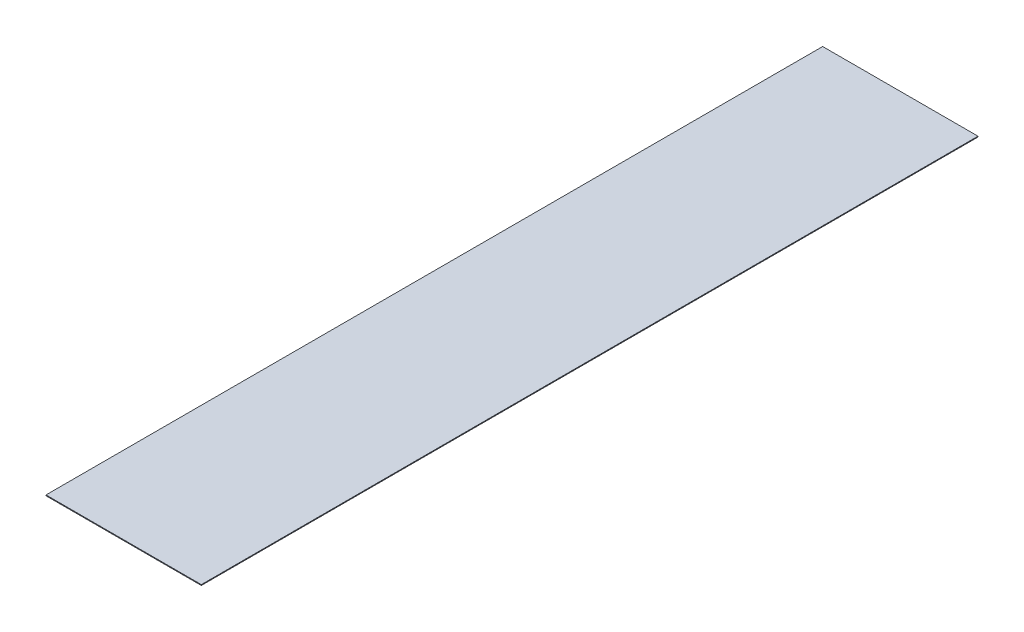
from build123d import *

# Parameters (mm, degrees)
SKETCH1_W           = 200
SKETCH1_H           = 1000
BOSS_EXTRUDE1_DEPTH = 1


with BuildPart() as part:
    # Sketch1 → Boss-Extrude1 (new body)
    with BuildSketch(Plane(origin=(0, 0, 0), x_dir=(1, 0, 0), z_dir=(0, 1, 0))):
        Rectangle(SKETCH1_W, SKETCH1_H)
    extrude(amount=BOSS_EXTRUDE1_DEPTH)


solid = part.part
